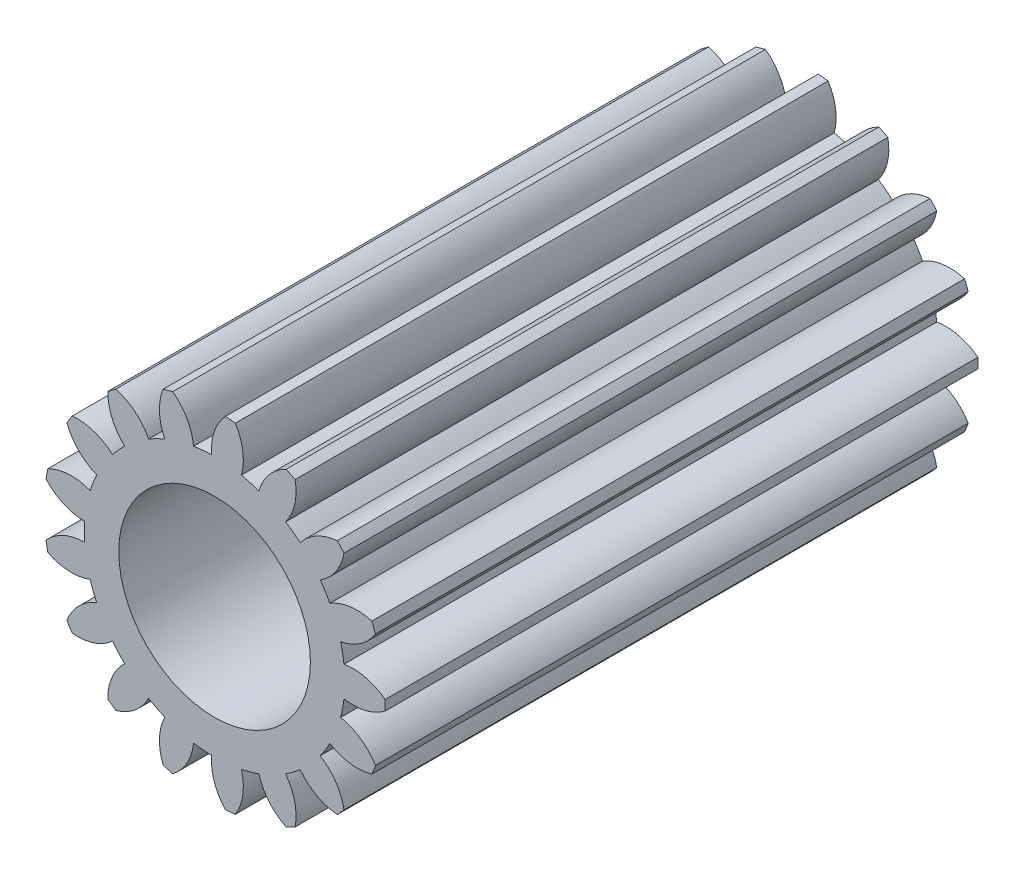
from build123d import *

# Parameters (mm, degrees)
SKETCH1_R           = 10.875
SKETCH1_R_2         = 8
BOSS_EXTRUDE1_DEPTH = 49.5
BOSS_EXTRUDE2_START = -49.5
BOSS_EXTRUDE2_DEPTH = 49.5
CIRPATTERN1_COUNT   = 17


with BuildPart() as part:
    # Sketch1 → Boss-Extrude1 (new body)
    with BuildSketch(Plane.XY):
        Circle(SKETCH1_R)
        Circle(SKETCH1_R_2, mode=Mode.SUBTRACT)
    extrude(amount=BOSS_EXTRUDE1_DEPTH)

    # Sketch2 → Boss-Extrude2 (add)
    with BuildSketch(Plane.XY.offset(49.5).offset(BOSS_EXTRUDE2_START)):
        with BuildLine():
            ThreePointArc((2.239420157, 10.641927568), (2.356131909, 12.447246966), (1.730141322, 14.144578856))
            ThreePointArc((1.730141322, 14.144578856), (1.314824122, 14.189212012), (0.898377166, 14.221653155))
            ThreePointArc((0.898377166, 14.221653155), (-0.028838658, 12.668247034), (-0.245840713, 10.872220902))
            ThreePointArc((-0.245840713, 10.872220902), (1.003418409, 10.828609167), (2.239420157, 10.641927568))
        make_face()
    boss_extrude2 = extrude(amount=BOSS_EXTRUDE2_DEPTH)

    # CirPattern1: Boss-Extrude2 ×17 about axis
    cirpattern1_axis = Axis((0, 0, 0), (0, 0, 1))
    for i in range(1, CIRPATTERN1_COUNT):
        add(boss_extrude2.rotate(cirpattern1_axis, i * 360 / CIRPATTERN1_COUNT))


solid = part.part
